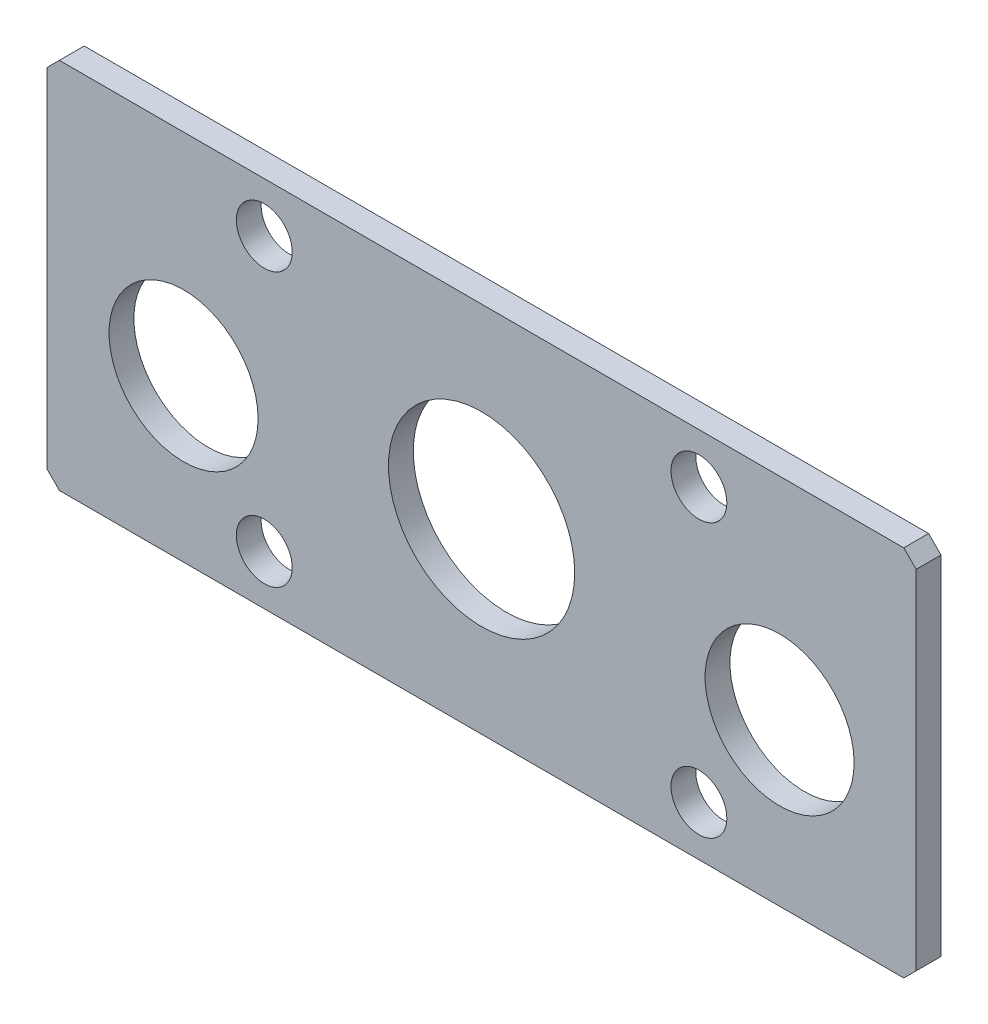
from build123d import *

# Parameters (mm, degrees)
SKETCH1_W                  = 70
SKETCH1_H                  = 30
SKETCH1_R                  = 6
SKETCH1_R_2                = 7.5
BOSS_EXTRUDE1_DEPTH        = 2
F_4_5_4_5_DIAMETER_HOLE1_D = 4.5
CHAMFER1_SIZE              = 1


with BuildPart() as part:
    # Sketch1 → Boss-Extrude1 (new body)
    with BuildSketch(Plane.XY):
        with Locations((0, 15)):
            Rectangle(SKETCH1_W, SKETCH1_H)
        with Locations((-24, 13)):
            Circle(SKETCH1_R, mode=Mode.SUBTRACT)
        with Locations((24, 13)):
            Circle(SKETCH1_R, mode=Mode.SUBTRACT)
        with Locations((0, 15)):
            Circle(SKETCH1_R_2, mode=Mode.SUBTRACT)
    extrude(amount=BOSS_EXTRUDE1_DEPTH)

    # Ø4.5 (4.5) Diameter Hole1 (through all)
    with Locations(Plane.XY.offset(2)):
        with Locations((-17.5, 26), (17.5, 26), (-17.5, 4), (17.5, 4)):
            Hole(F_4_5_4_5_DIAMETER_HOLE1_D / 2)

    # Chamfer1
    chamfer1_edges = [part.edges().sort_by_distance(p)[0] for p in [
        (35, 0, 1),
        (-35, 0, 1),
        (-35, 30, 1),
        (35, 30, 1),
    ]]
    chamfer(chamfer1_edges, length=CHAMFER1_SIZE)


solid = part.part
